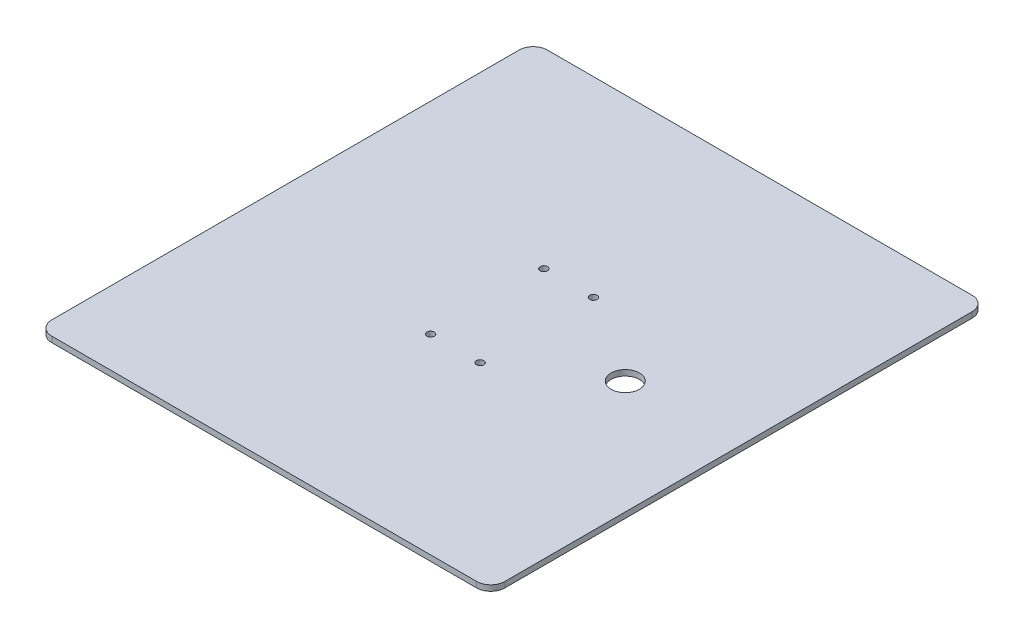
from build123d import *

# Parameters (mm, degrees)
SKETCH1_W                      = 320
SKETCH1_H                      = 350
BOSS_EXTRUDE1_DEPTH            = 4
F_5_2_5_2_DIAMETER_HOLE1_D     = 5.2
F_5_2_5_2_DIAMETER_HOLE1_DEPTH = 10.1
F_5_2_5_2_DIAMETER_HOLE1_TIP   = 1.562237609
FILLET1_R                      = 10
SKETCH4_R                      = 10
CUT_EXTRUDE1_DEPTH             = 238.151850088


with BuildPart() as part:
    # Sketch1 → Boss-Extrude1 (new body)
    with BuildSketch(Plane(origin=(0, 0, 0), x_dir=(1, 0, 0), z_dir=(0, 1, 0))):
        Rectangle(SKETCH1_W, SKETCH1_H)
    extrude(amount=BOSS_EXTRUDE1_DEPTH)

    # Ø5.2 (5.2) Diameter Hole1
    with Locations(Plane(origin=(0, 4, 0), x_dir=(1, 0, 0), z_dir=(0, 1, 0))):
        with Locations((-17.5, 40), (17.5, -40), (-17.5, -40), (17.5, 40)):
            Hole(F_5_2_5_2_DIAMETER_HOLE1_D / 2, depth=F_5_2_5_2_DIAMETER_HOLE1_DEPTH)
            with Locations((0, 0, -(F_5_2_5_2_DIAMETER_HOLE1_DEPTH + F_5_2_5_2_DIAMETER_HOLE1_TIP / 2))):  # 118° drill point
                Cone(0, F_5_2_5_2_DIAMETER_HOLE1_D / 2, F_5_2_5_2_DIAMETER_HOLE1_TIP, mode=Mode.SUBTRACT)

    # Fillet1
    fillet1_edges = [part.edges().sort_by_distance(p)[0] for p in [
        (-160, 2, -175),
        (160, 2, -175),
        (160, 2, 175),
        (-160, 2, 175),
    ]]
    fillet(fillet1_edges, radius=FILLET1_R)

    # Sketch4 → Cut-Extrude1 (cut, through all)
    with BuildSketch(Plane(origin=(0, 4, 0), x_dir=(1, 0, 0), z_dir=(0, 1, 0))):
        with Locations(Location((80, 0, 0), (0, 0, 270))):
            Circle(SKETCH4_R)
    extrude(amount=-CUT_EXTRUDE1_DEPTH, mode=Mode.SUBTRACT)


solid = part.part
